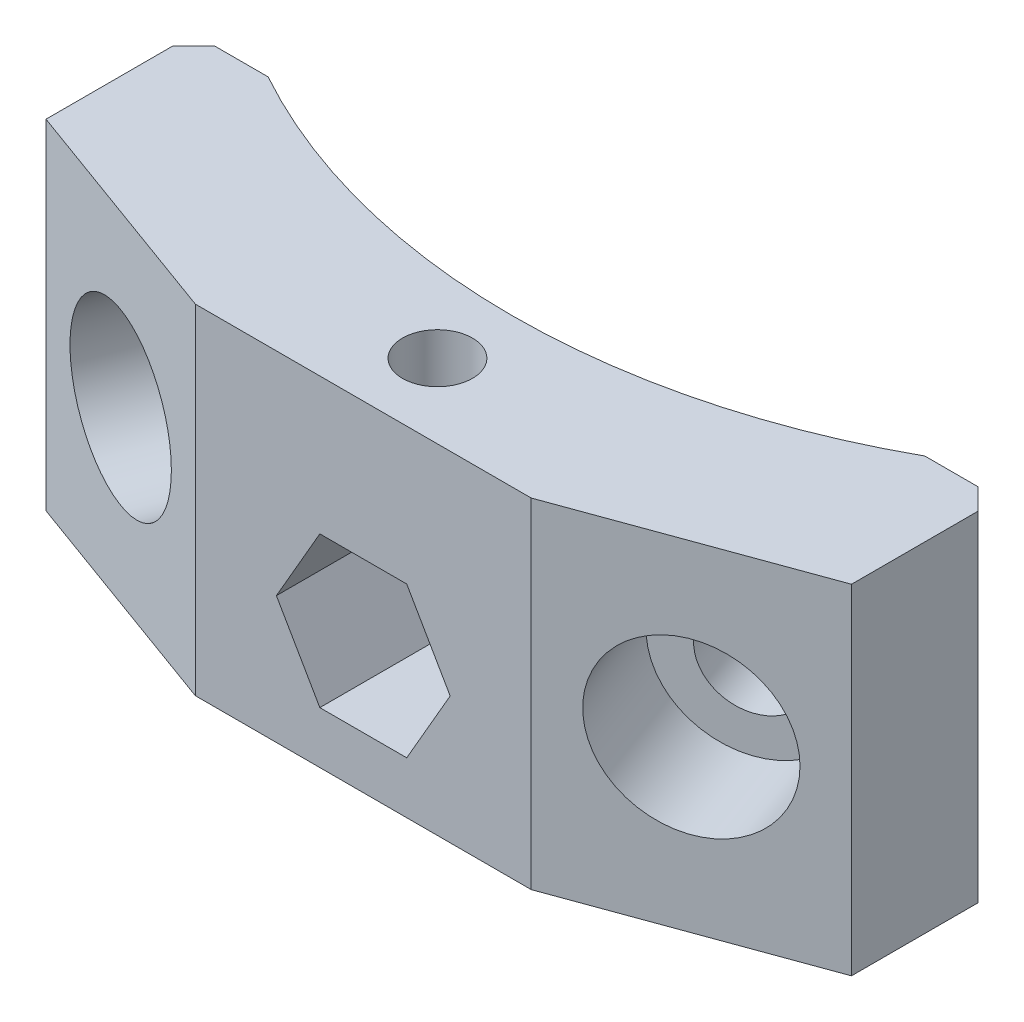
SolidWorks part; units mm, degrees
material "45"
ref_plane "Front Plane" through (0, 0, 0) normal (0, 0, 1) x (1, 0, 0)
ref_plane "Top Plane" through (0, 0, 0) normal (0, 1, 0) x (1, 0, 0)
ref_plane "Right Plane" through (0, 0, 0) normal (1, 0, 0) x (0, 0, -1)
sketch "Sketch1" plane through (0, 0, 0) normal (0, 1, 0) x (1, 0, 0)
  line L0 (0, -32) -> (0, -45.8587) construction
  line L1 (-7.9221, -39) -> (7.9221, -39)
  line L2 (7.9221, -39) -> (19, -34.968)
  line L3 (-19, -28) -> (-19, -34.968)
  line L4 (19, -28) -> (19, -34.968)
  line L5 (-7.9221, -39) -> (-19, -34.968)
  line L6 (-13.4611, -36.984) -> (0, 0) construction
  line L7 (13.4611, -36.984) -> (0, 0) construction
  line L8 (-19, -28) -> (-15.4919, -28)
  line L9 (19, -28) -> (15.4919, -28)
  arc A1 (-15.4919, -28) -> (15.4919, -28) centre (0, 0) ccw
  dimension "D2" = 64
  dimension "D1" = 7
  dimension "D3" = 38
  dimension "D4" = 40
  dimension "D5" = 11
extrude "Boss-Extrude1" add sketch "Sketch1" along normal mid plane 16
sketch "Sketch2" plane through (0, 0, 39) normal (0, 0, 1) x (1, 0, 0)
  line L1 (4.0992, -2) -> (2.0496, 1.55)
  line L2 (2.0496, 1.55) -> (-2.0496, 1.55)
  line L3 (-2.0496, 1.55) -> (-4.0992, -2)
  line L4 (-4.0992, -2) -> (-2.0496, -5.55)
  line L5 (-2.0496, -5.55) -> (2.0496, -5.55)
  line L6 (2.0496, -5.55) -> (4.0992, -2)
  line L7 (-7.9221, -8) -> (7.9221, -8) construction
  circle A0 centre (0, -2) radius 3.55 construction
  dimension "D1" = 7.1
  dimension "D2" = 6
extrude "Cut-Extrude2" cut sketch "Sketch2" against normal through all
hole_wizard "M4 Tapped Hole1" positions "Sketch5" profile "Sketch4" tap size "M4" standard "GB"
sketch "Sketch5" plane through (0, 8, 0) normal (0, 1, 0) x (1, 0, 0)
  line L0 (0, -32) -> (0, -39) construction
  line L3 (-7.9221, -39) -> (7.9221, -39) construction
  arc A0 (-15.4919, -28) -> (15.4919, -28) centre (0, 0) ccw construction
  point P0 (0, -35.5)
sketch "Sketch4" plane through (0, 8, 35.5) normal (1, 0, 0) x (0, 0, 1)
  line L0 (0, 0) -> (0, 12.4914)
  line L1 (0, 12.4914) -> (1.65, 11.5)
  line L2 (1.65, 11.5) -> (1.65, 0)
  line L5 (1.65, 0) -> (0, 0)
  line L10 (0, 12.4914) -> (-1.65, 11.5) construction
  line L11 (0, -6.35) -> (0, 107.95) construction
  dimension "螺纹孔钻头直径" = 3.3
  dimension "螺纹孔钻头深度" = 11.5
  dimension "导头角度" = 118
cosmetic thread "Hole thread 1" parameters "D1"=7.4, "D2"=4
hole_wizard "Hole size per socket head cap screw type 2" positions "Sketch10" profile "Sketch9" counterbore size "M4" standard "GB" end condition through all
sketch "Sketch10" plane through (-13.4611, 0, 36.984) normal (-0.342, 0, 0.9397) x (0.9397, 0, 0.342)
  point P0 (0, 0)
sketch "Sketch9" plane through (-13.4611, 0, 36.984) normal (0, 1, 0) x (0.9397, 0, 0.342)
  line L0 (0, 0) -> (0, 19.5445)
  line L1 (0, 19.5445) -> (2.25, 19.5445)
  line L3 (2.25, 19.5445) -> (2.25, 5)
  line L4 (2.25, 5) -> (4, 5)
  line L5 (4, 5) -> (4, 0)
  line L7 (4, 0) -> (0, 0)
  line L11 (0, -6.35) -> (0, 107.95) construction
  dimension "通孔孔直径" = 4.5
  dimension "通孔孔深度" = 19.5445
  dimension "柱形沉头孔直径" = 8
  dimension "柱形沉头孔深度" = 5
mirror "Mirror3" about plane through (0, 0, 0) normal (1, 0, 0) of "Hole size per socket head cap screw type 2"
chamfer "Chamfer2" distance 1 angle 45 2 edges at (19, 0, 28) (-19, 0, 28)
